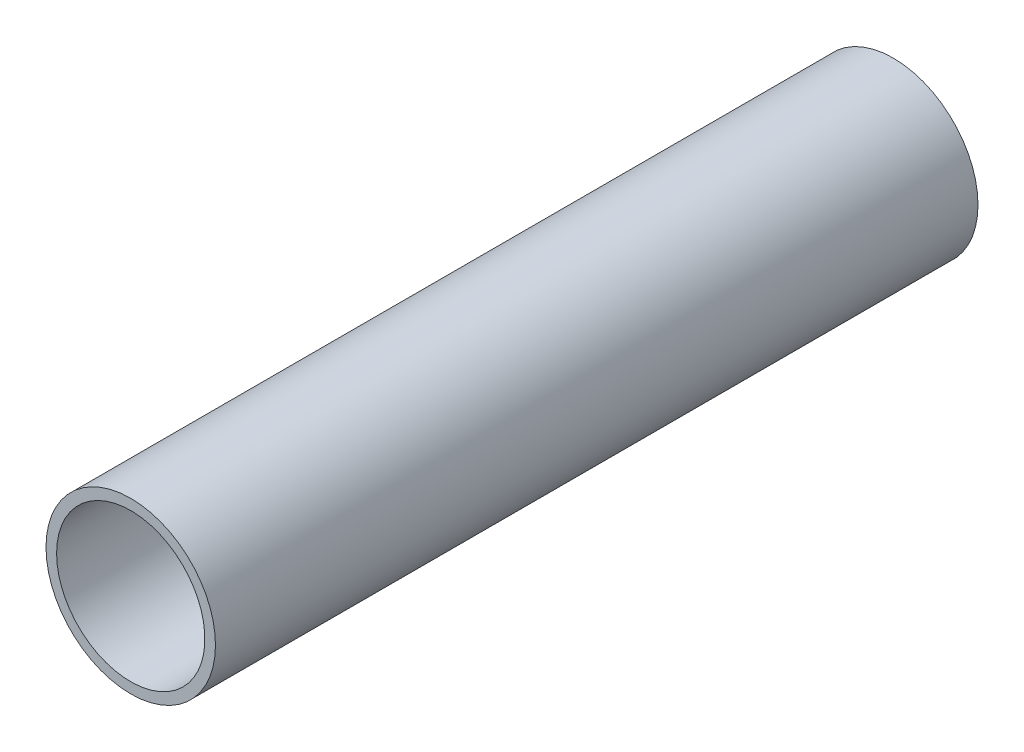
from build123d import *

# Parameters (mm, degrees)
SKETCH_1_R      = 40
SKETCH_1_R_2    = 35
EXTRUDE_1_DEPTH = 360


with BuildPart() as part:
    # 草图1 → 凸台-拉伸1 (new body)
    with BuildSketch(Plane.XY):
        with Locations(Location((0, 0, 0), (0, 0, 180))):
            Circle(SKETCH_1_R)
        with Locations(Location((0, 0, 0), (0, 0, 180))):
            Circle(SKETCH_1_R_2, mode=Mode.SUBTRACT)
    extrude(amount=EXTRUDE_1_DEPTH)


solid = part.part
